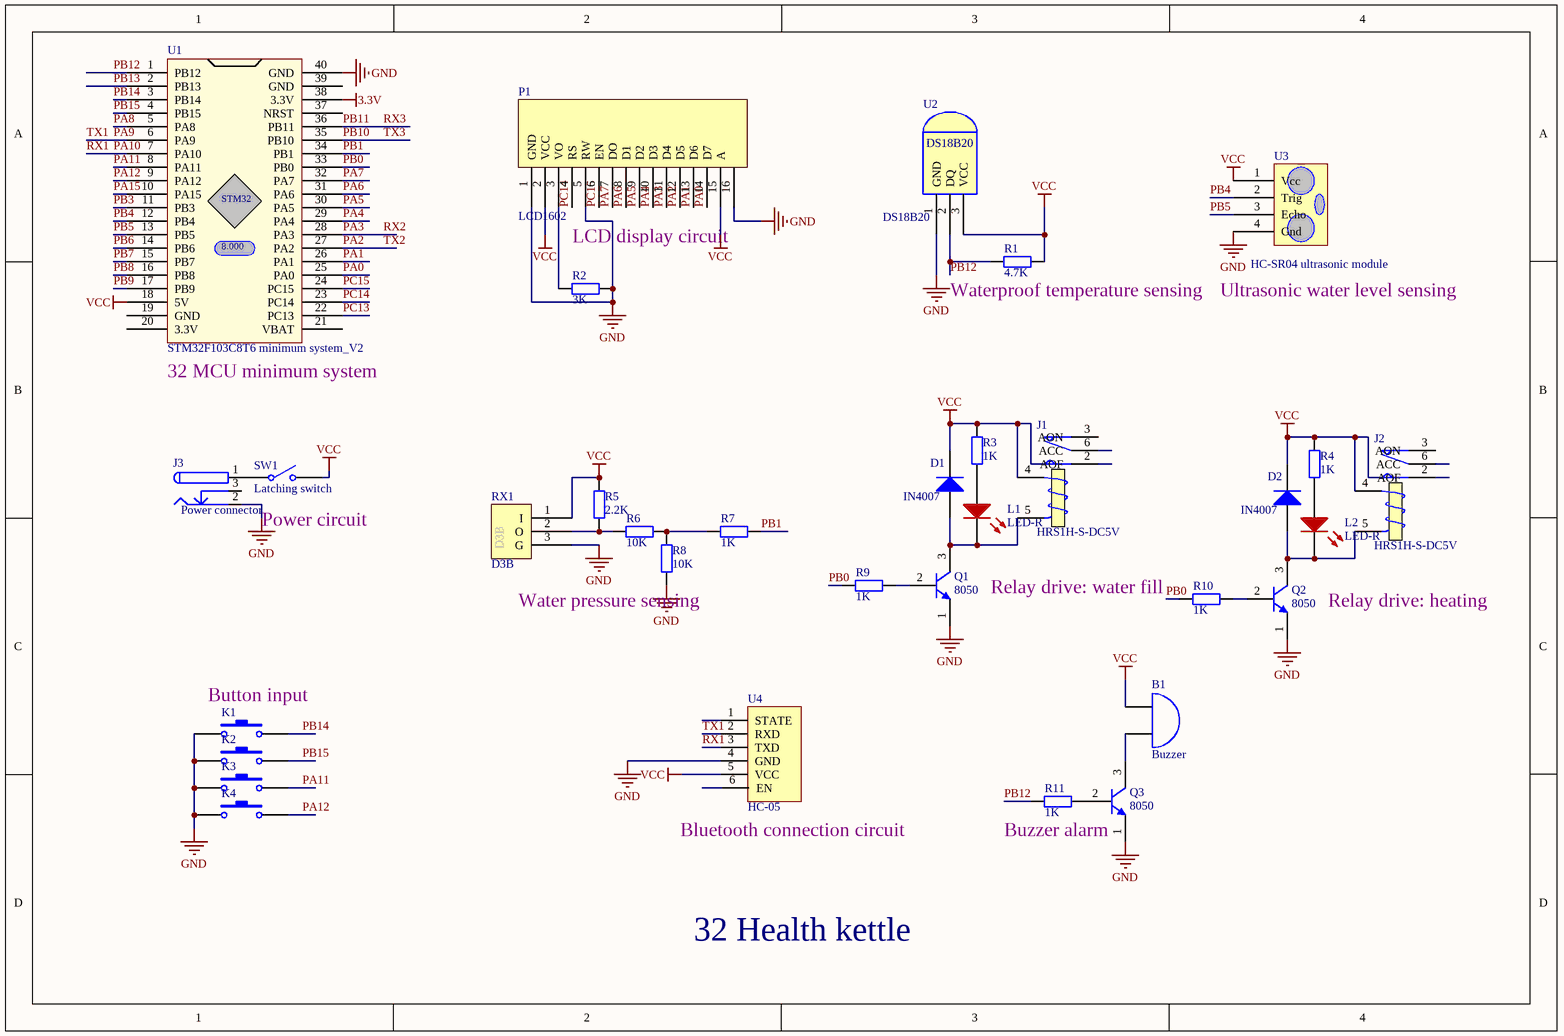
[diagram p0: MISC84237-2.SchDoc]
# Altium project MISC84237.PrjPcb
5 sheets, 81 parts. Net scope: global (net labels, ports and power ports of the same name join across sheets).
Board files: MISC84237-4.PcbDoc, MISC84237-7.PcbDoc, MISC84237.PcbDoc
Sheets:
  MISC84237-2.SchDoc
  MISC84237-3.SchDoc
  MISC84237-5.SchDoc
  MISC84237-6.SchDoc
  MISC84237-8.SchDoc

## Sheet MISC84237-2.SchDoc
size A4; PageSetup: Record=PageOptions|CenterHorizontal=True|CenterVertical=True|PrintScale=0.97|XCorrection=1.00|YCorrection=1.00|PrintKind=0|BorderSize=5000000|LeftOffset=0|BottomOffset=0|Orientation=2|PaperLength=1000|PaperWidth=1000|Scale=100|PaperSource=7|PrintQuality=-4|MediaType=1|DitherType=10|PaperKind=A4|PrintScaleMode=1

### Parts
(Parts that share a designator on the sheet are numbered #1, #2 ... from top to bottom, then left to right.)
B1  Buzzer  [Buzzy-Small]
D1#1  IN4007  [Diode-0.3]
D2#1  IN4007  [Diode-0.3]
J1#1  HRS1H-S-DC5V  [JDIANQI]
J2#1  HRS1H-S-DC5V  [JDIANQI]
J3#1  Power connector  [DC-JACK]
K1#1  Tactile button  [SW-6-6]  (value not drawn)
K2#1  Tactile button  [SW-6-6]  (value not drawn)
K3#1  Tactile button  [SW-6-6]  (value not drawn)
K4#1  Tactile button  [SW-6-6]  (value not drawn)
L1#1  LED-R  [LED-3]
L2#1  LED-R  [LED-3]
P1#1  LCD1602  [1602]
Q1#1  8050  [TO-92-2N3906]
Q2#1  8050  [TO-92-2N3906]
Q3#1  8050  [TO-92-2N3906]
R1#1  4.7K  [AXIAL-0.3]
R2#1  3K  [AXIAL-0.3]
R3#1  1K  [AXIAL-0.3]
R4#1  1K  [AXIAL-0.3]
R5#1  2.2K  [AXIAL-0.3]
R6#1  10K  [AXIAL-0.3]
R7#1  1K  [AXIAL-0.3]
R8#1  10K  [AXIAL-0.3]
R9#1  1K  [AXIAL-0.3]
R10#1  1K  [AXIAL-0.3]
R11#1  1K  [AXIAL-0.3]
RX1#1  D3B  [HDR1X3]
SW1#1  Latching switch  [SW1]
U1#1  STM32F103C8T6 minimum system_V2  [STM32F103C8T6_V2]
U2#1  DS18B20  [DS18b20]
U3#1  HC-SR04 ultrasonic module  [chaoshengbo-4]
U4#1  HC-05  [bluetooth]

### Nets
3.3V: U1#1.38(3.3V)
GND: J3#1.2 K1#1.1 K2#1.1 K3#1.1 K4#1.1 P1#1.1(GND) P1#1.5(RW) P1#1.16(K) Q1#1.1(E) Q2#1.1(E) Q3#1.1(E) R2#1.2 R8#1.1 RX1#1.3(G) U1#1.40(GND) U2#1.1(GND) U3#1.4(Gnd) U4#1.4(GND)
VCC: B1.1(A) D1#1.2(K) D2#1.2(K) J1#1.4(T1) J2#1.4(T1) P1#1.2(VCC) P1#1.15(A) R1#1.2 R3#1.2 R4#1.2 R5#1.2 RX1#1.1(I) SW1#1.2(NO) U1#1.18(5V) U2#1.3(VCC) U3#1.1(Vcc) U4#1.5(VCC)
PA0: P1#1.14(D7) U1#1.25(PA0)
PA1: P1#1.13(D6) U1#1.26(PA1)
PA2: P1#1.12(D5) U1#1.27(PA2)  [also labelled TX2]
PA3: P1#1.11(D4) U1#1.28(PA3)  [also labelled RX2]
PA4: P1#1.10(D3) U1#1.29(PA4)
PA5: P1#1.9(D2) U1#1.30(PA5)
PA6: P1#1.8(D1) U1#1.31(PA6)
PA7: P1#1.7(DO) U1#1.32(PA7)
PA8: U1#1.5(PA8)
PA9: U1#1.6(PA9) U4#1.2(RXD)  [also labelled TX1]
PA10: U1#1.7(PA10) U4#1.3(TXD)  [also labelled RX1]
PA11: K3#1.2 U1#1.8(PA11)
PA12: K4#1.2 U1#1.9(PA12)
PA15: U1#1.10(PA15)
PB0: R9#1.1 R10#1.1 U1#1.33(PB0)
PB1: R7#1.1 U1#1.34(PB1)
PB3: U1#1.11(PB3)
PB4: U1#1.12(PB4) U3#1.2(Trig)
PB5: U1#1.13(PB5) U3#1.3(Echo)
PB6: U1#1.14(PB6)
PB7: U1#1.15(PB7)
PB8: U1#1.16(PB8)
PB9: U1#1.17(PB9)
PB10: U1#1.35(PB10)  [also labelled TX3]
PB11: U1#1.36(PB11)  [also labelled RX3]
PB12: R1#1.1 R11#1.1 U1#1.1(PB12) U2#1.2(DQ)
PB13: U1#1.2(PB13)
PB14: K1#1.2 U1#1.3(PB14)
PB15: K2#1.2 U1#1.4(PB15)
PC13: U1#1.22(PC13)
PC14: P1#1.4(RS) U1#1.23(PC14)
PC15: P1#1.6(EN) U1#1.24(PC15)
NetB1_2: B1.2(B) Q3#1.3(C)
NetD1#1_1: D1#1.1(A) J1#1.5(T2) L1#1.2(K) Q1#1.3(C)
NetD2#1_1: D2#1.1(A) J2#1.5(T2) L2#1.2(K) Q2#1.3(C)
NetJ3#1_1: J3#1.1 SW1#1.1(COMMON)
NetL1#1_1: L1#1.1(A) R3#1.1
NetL2#1_1: L2#1.1(A) R4#1.1
NetP1#1_3: P1#1.3(VO) R2#1.1
NetQ1#1_2: Q1#1.2(B) R9#1.2
NetQ2#1_2: Q2#1.2(B) R10#1.2
NetQ3#1_2: Q3#1.2(B) R11#1.2
NetR5#1_1: R5#1.1 R6#1.1 RX1#1.2(O)
NetR6#1_2: R6#1.2 R7#1.2 R8#1.2

Not connected (* = marked no-connect by the designer): J1#1 2(AOF) 3(AON) 6(ACC); J2#1 2(AOF) 3(AON) 6(ACC); J3#1 3; U1#1 19(GND) 20(3.3V) 21(VBAT) 37(NRST) 39(GND); U4#1 1(STATE) 6(EN)

### Notes on the sheet
- LCD display circuit
- (near R1#1) Waterproof temperature sensing
- (near U3#1) Ultrasonic water level sensing
- (near U1#1) 32 MCU minimum system
- Power circuit
- (near R8#1) Water pressure sensing
- (near R10#1) Relay drive: water fill
- Relay drive: heating
- (near K1#1) Button input
- (near U4#1) Bluetooth connection circuit
- (near Q3#1) Buzzer alarm
- 32 Health kettle

### Library data of the parts
B1 = Bell: Electrical Bell; Value: 5V  有源蜂鸣器; Published: 24-Mar-1999; LatestRevisionDate: 17-Jul-2002; LatestRevisionNote: Re-released for DXP Platform.; PackageReference: PIN2; Publisher: Altium Limited
D1#1 D2#1 = DIODE: Value: IN4007二极管
J1#1 J2#1 = jidianqi: Value: HK4100F-DC5V-SHG 继电器（5V黄色6腿继电器）
J3#1 = DC002: Low Voltage Power Supply Connector; Value: DC-002电源插座 3.5-1.1MM DC电源座; Published: 17-Dec-2003; DatasheetDocument: 09-May-2002; ComponentLink1Description: Manufacturer Link; ComponentLink1URL: http://domino.kycon.com/internet/Products.html; Publisher: Altium Limited
K1#1 K2#1 K3#1 K4#1 = SW-AJ: Value: 轻触按键
L1#1 L2#1 = LED-R: Value: 3mm红色LED灯
P1#1 = LCD1602: Value: LCD1602液晶显示+16P排座
Q1#1 Q2#1 Q3#1 = 8050: Value: 8050三极管
R1#1 = RES2: Resistor; Value: 4.7K电阻
R2#1 = Res2: Resistor; Value: 3K电阻
R3#1 R4#1 = Res2: Resistor; Value: 1K电阻
R5#1 = RES2: Resistor; Value: 2.2K电阻
R6#1 R8#1 = RES2: Resistor; Value: 10K电阻
R7#1 = RES0.4: Value: 1K电阻
R9#1 R10#1 R11#1 = RES2: Resistor; Value: 1K电阻
RX1#1 = D3B: Value: D3B压力传感器+瓶盖
SW1#1 = SW-SPST: Value: 自锁开关
U1#1 = STM32F103C8T6最小系统_V2
U2#1 = DS18B20: Value: 防水DS18B20温度传感器
U3#1 = HC-SR04: Value: HC-SR04  超声波模块
U4#1 = Bluetooth: Value: 蓝牙 HC-05模块+6P排座

## Sheet MISC84237-3.SchDoc
size A3; PageSetup: Record=PageOptions¦CenterHorizontal=True¦CenterVertical=True¦PrintScale=0.97¦XCorrection=1.00¦YCorrection=1.00¦PrintKind=0¦BorderSize=5000000¦LeftOffset=0¦BottomOffset=0¦Orientation=2¦PaperLength=1000¦PaperWidth=1000¦Scale=100¦PaperSource=7¦PrintQuality=-4¦MediaType=1¦DitherType=10¦PaperKind=A4¦PrintScaleMode=1
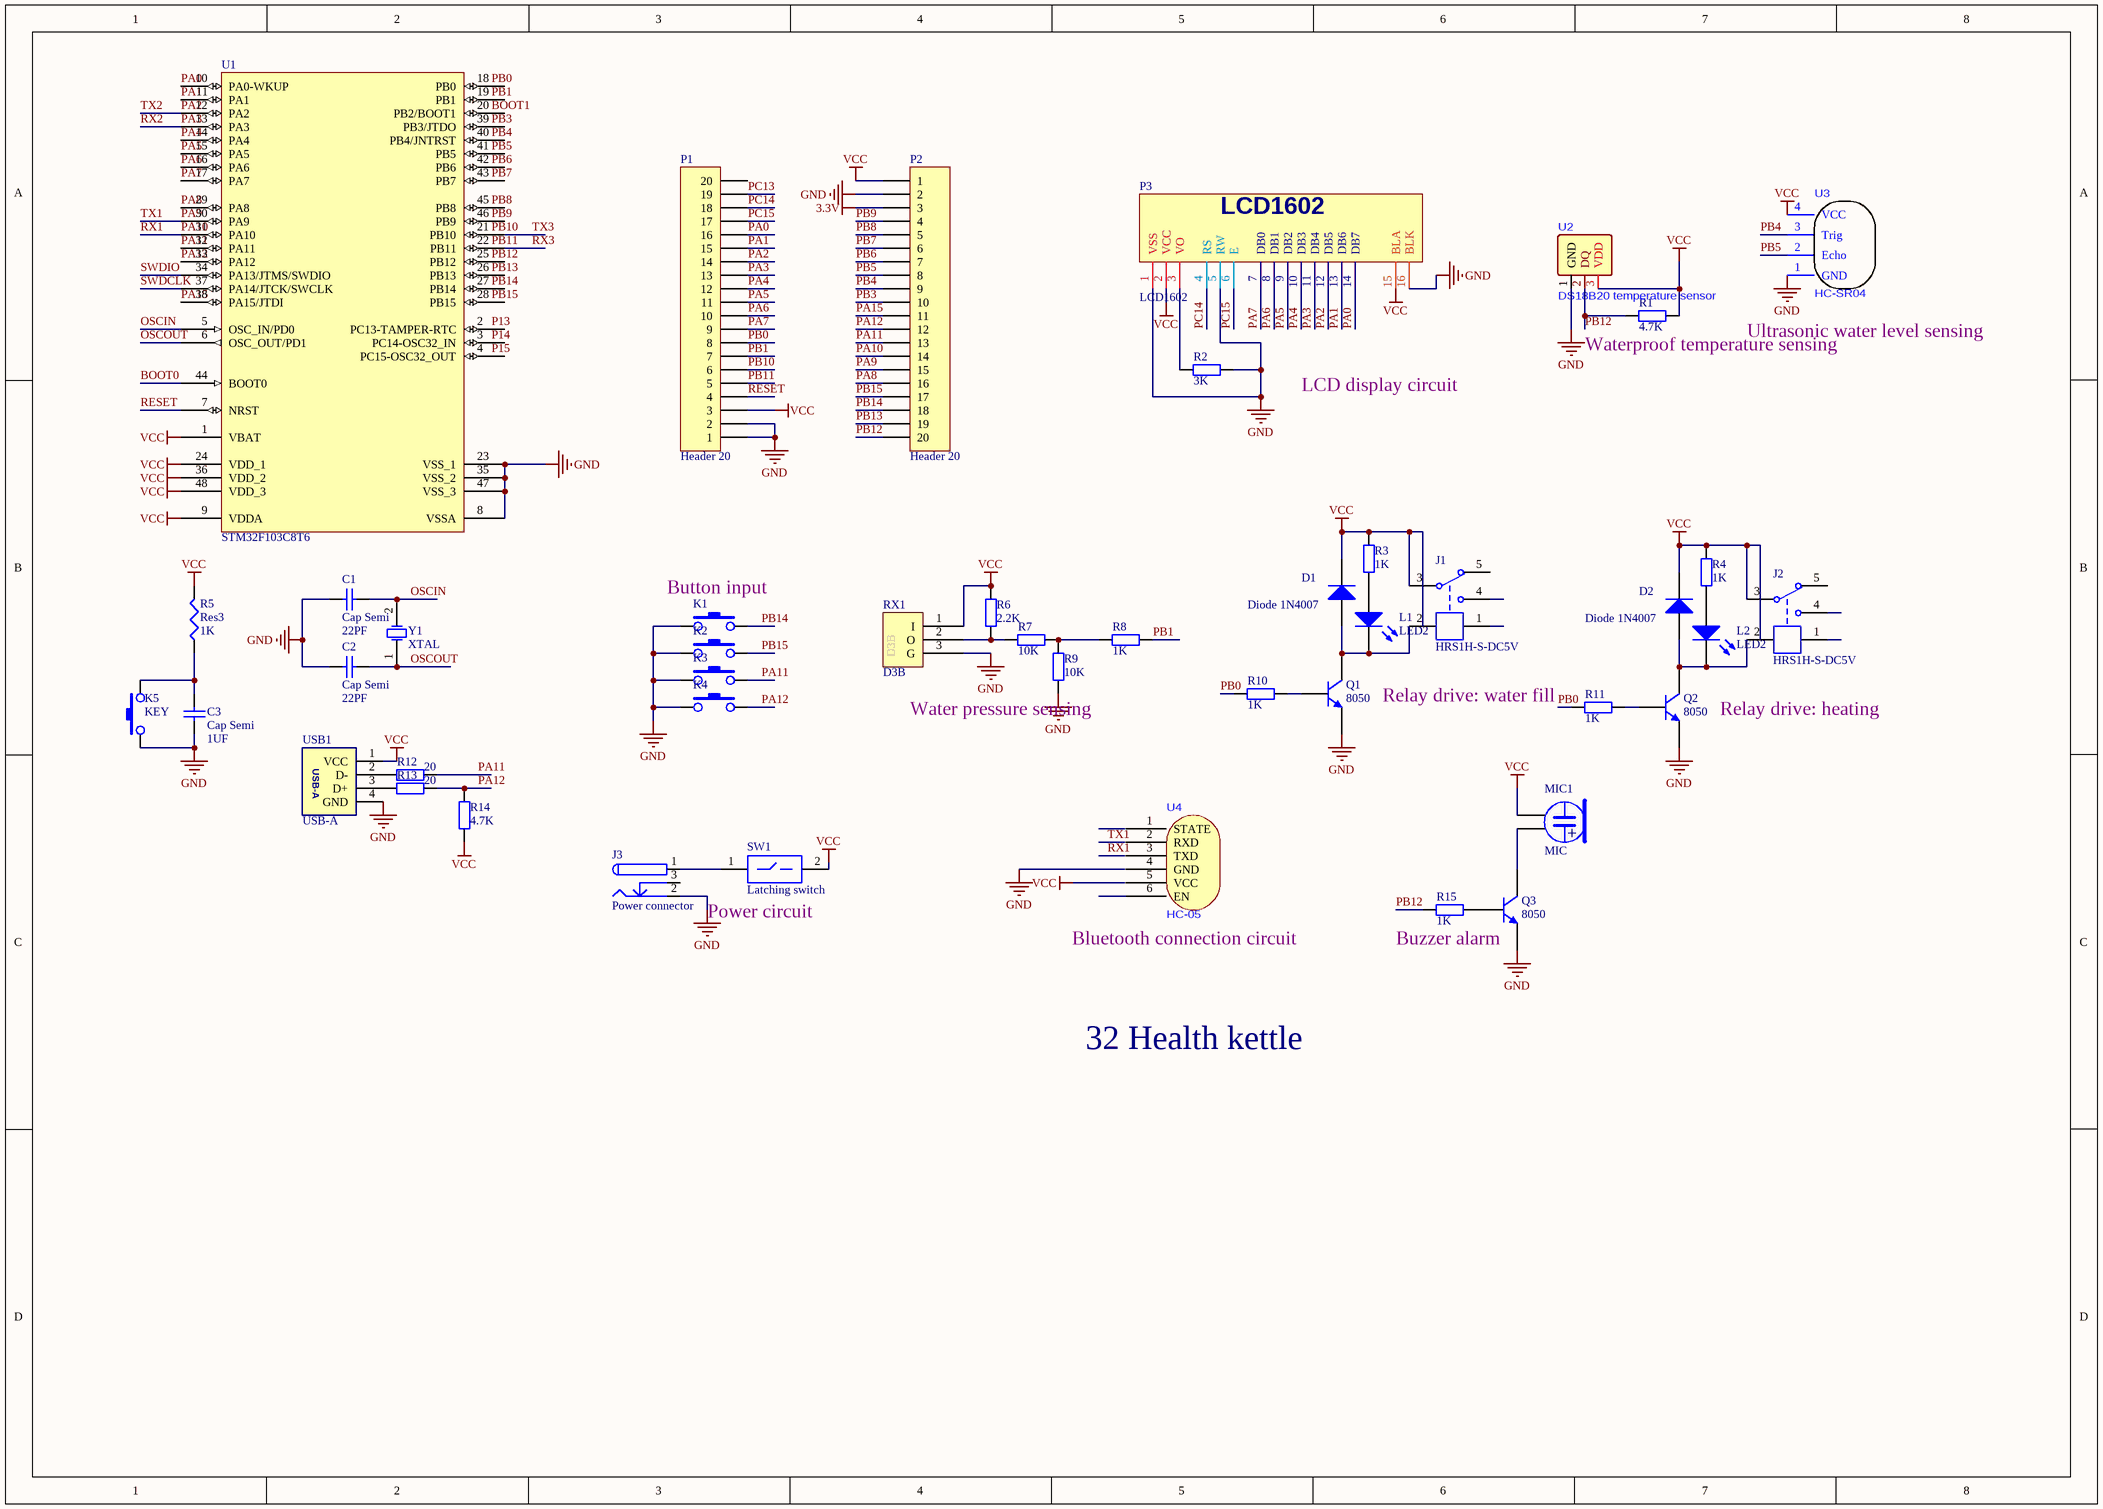
[diagram p1: MISC84237-3.SchDoc]

### Parts
(Parts that share a designator on the sheet are numbered #1, #2 ... from top to bottom, then left to right.)
C1  Cap Semi  value 22PF  [C1206]
C2  Cap Semi  value 22PF  [C1206]
C3  Cap Semi  value 1UF  [C1206]
D1#2  Diode 1N4007  [DO-41]
D2#2  Diode 1N4007  [DO-41]
J1#2  HRS1H-S-DC5V  [HRS1H]
J2#2  HRS1H-S-DC5V  [HRS1H]
J3#2  Power connector  [DC-002]
K1#2  KEY  [DIP-3X6X4.3]  (value not drawn)
K2#2  KEY  [DIP-3X6X4.3]  (value not drawn)
K3#2  KEY  [DIP-3X6X4.3]  (value not drawn)
K4#2  KEY  [DIP-3X6X4.3]  (value not drawn)
K5  KEY  [DIP-3X6X4.3]
L1#2  LED2  [3.2X1.6X1.1]
L2#2  LED2  [3.2X1.6X1.1]
MIC1  MIC  [MIC-4.5X1.9]
P1#2  Header 20  [HDR1X20]
P2  Header 20  [HDR1X20]
P3  LCD1602  [LCD1602]
Q1#2  8050  [TO-226-AA]
Q2#2  8050  [TO-226-AA]
Q3#2  8050  [TO-226-AA]
R1#2  4.7K  [AXIAL-0.3]
R2#2  3K  [AXIAL-0.3]
R3#2  1K  [AXIAL-0.3]
R4#2  1K  [AXIAL-0.3]
R5#2  Res3  value 1K  [J1-0603]
R6#2  2.2K  [AXIAL-0.3]
R7#2  10K  [AXIAL-0.3]
R8#2  1K  [AXIAL-0.3]
R9#2  10K  [AXIAL-0.3]
R10#2  1K  [AXIAL-0.3]
R11#2  1K  [AXIAL-0.3]
R12  20  [AXIAL-0.3]
R13  20  [AXIAL-0.3]
R14  4.7K  [AXIAL-0.3]
R15  1K  [AXIAL-0.3]
RX1#2  D3B  [HDR1X3]
SW1#2  Latching switch  [DIP-1P]
U1#2  STM32F103C8T6  [LQFP48_N]
U2#2  DS18B20 temperature sensor  [DS18B20温度传感器]
U3#2  HC-SR04  [HC-SR04]
U4#2  HC-05  [HC-05]
USB1  USB-A  [USB-A/S_A]
Y1  XTAL  [R38]

### Nets
3.3V: P2.3
GND: C1.2 C2.2 C3.1 J3#2.2 K1#2.1 K2#2.1 K3#2.1 K4#2.1 K5.1 P1#2.1 P1#2.2 P2.2 P3.1(VSS) P3.5(RW) P3.16(BLK) Q1#2.3(E) Q2#2.3(E) Q3#2.3(E) R2#2.2 R9#2.1 RX1#2.3(G) U1#2.8(VSSA) U1#2.23(VSS_1) U1#2.35(VSS_2) U1#2.47(VSS_3) U2#2.1(GND) U3#2.1(GND) USB1.4(GND)
VCC: D1#2.2(K) D2#2.2(K) J1#2.3 J2#2.3 MIC1.2 P1#2.3 P2.1 P3.2(VCC) P3.15(BLA) R1#2.2 R3#2.2 R4#2.2 R5#2.2 R6#2.2 R14.2 RX1#2.1(I) SW1#2.2 U1#2.1(VBAT) U1#2.9(VDDA) U1#2.24(VDD_1) U1#2.36(VDD_2) U1#2.48(VDD_3) U2#2.3(VDD) U3#2.4(VCC) USB1.1(VCC)
BOOT0: U1#2.44(BOOT0)
OSCIN: C1.1 U1#2.5(OSC_IN/PD0) Y1.2(OSC2)
OSCOUT: C2.1 U1#2.6(OSC_OUT/PD1) Y1.1(OSC1)
PA0: P1#2.16 P3.14(DB7) U1#2.10(PA0-WKUP)
PA1: P1#2.15 P3.13(DB6) U1#2.11(PA1)
PA2: P1#2.14 P3.12(DB5) U1#2.12(PA2)  [also labelled TX2]
PA3: P1#2.13 P3.11(DB4) U1#2.13(PA3)  [also labelled RX2]
PA4: P1#2.12 P3.10(DB3) U1#2.14(PA4)
PA5: P1#2.11 P3.9(DB2) U1#2.15(PA5)
PA6: P1#2.10 P3.8(DB1) U1#2.16(PA6)
PA7: P1#2.9 P3.7(DB0) U1#2.17(PA7)
PA8: P2.16 U1#2.29(PA8)
PA9: P2.15 U1#2.30(PA9)  [also labelled TX1]
PA10: P2.14 U1#2.31(PA10)  [also labelled RX1]
PA11: K3#2.3 P2.13 R12.1 U1#2.32(PA11)
PA12: K4#2.3 P2.12 R13.1 R14.1 U1#2.33(PA12)
PA15: P2.11 U1#2.38(PA15/JTDI)
PB0: P1#2.8 R10#2.1 R11#2.1
PB1: P1#2.7 R8#2.1
PB3: P2.10
PB4: P2.9 U3#2.3(Trig)
PB5: P2.8 U3#2.2(Echo)
PB6: P2.7
PB7: P2.6
PB8: P2.5
PB9: P2.4
PB10: P1#2.6 U1#2.21(PB10)  [also labelled TX3]
PB11: P1#2.5 U1#2.22(PB11)  [also labelled RX3]
PB12: P2.20 R1#2.1 R15.1 U2#2.2(DQ)
PB13: P2.19
PB14: K1#2.3 P2.18
PB15: K2#2.3 P2.17
PC13: P1#2.19
PC14: P1#2.18 P3.4(RS)
PC15: P1#2.17 P3.6(E)
RESET: P1#2.4 U1#2.7(NRST)
SWDCLK: U1#2.37(PA14/JTCK/SWCLK)
SWDIO: U1#2.34(PA13/JTMS/SWDIO)
NetC3_2: C3.2 K5.3 R5#2.1
NetD1#2_1: D1#2.1(A) J1#2.2 L1#2.2(K) Q1#2.1(C)
NetD2#2_1: D2#2.1(A) J2#2.2 L2#2.2(K) Q2#2.1(C)
NetJ3#2_1: J3#2.1 SW1#2.1(A1)
NetL1#2_1: L1#2.1(A) R3#2.1
NetL2#2_1: L2#2.1(A) R4#2.1
NetMIC1_1: MIC1.1 Q3#2.1(C)
NetP3_3: P3.3(VO) R2#2.1
NetQ1#2_2: Q1#2.2(B) R10#2.2
NetQ2#2_2: Q2#2.2(B) R11#2.2
NetQ3#2_2: Q3#2.2(B) R15.2
NetR6#2_1: R6#2.1 R7#2.1 RX1#2.2(O)
NetR7#2_2: R7#2.2 R8#2.2 R9#2.2
NetR12_2: R12.2 USB1.2(D-)
NetR13_2: R13.2 USB1.3(D+)

Not connected (* = marked no-connect by the designer): J1#2 1 4 5; J2#2 1 4 5; J3#2 3; P1#2 20; U1#2 2(PC13-TAMPER-RTC) 3(PC14-OSC32_IN) 4(PC15-OSC32_OUT) 18(PB0) 19(PB1) 20(PB2/BOOT1) 25(PB12) 26(PB13) 27(PB14) 28(PB15) 39(PB3/JTDO) 40(PB4/JNTRST) 41(PB5) 42(PB6) 43(PB7) 45(PB8) 46(PB9); U4#2 1(STATE) 2(RXD) 3(TXD) 4(GND) 5(VCC) 6(EN)

### Notes on the sheet
- (near R1#2) Waterproof temperature sensing
- (near U3#2) Ultrasonic water level sensing
- LCD display circuit
- (near K1#2) Button input
- (near R9#2) Water pressure sensing
- (near R11#2) Relay drive: water fill
- Relay drive: heating
- Power circuit
- (near U4#2) Bluetooth connection circuit
- (near Q3#2) Buzzer alarm
- 32 Health kettle
- Labels drawn without touching a wire or pin: BOOT1, P13, P14, P15, PB0, PB1, PB3, PB4, PB5, PB6, PB7, PB8, PB9, PB10, PB11, PB12, PB13, PB14, PB15

### Library data of the parts
C1-C3 = Cap Semi: Capacitor (Semiconductor SIM Model); Published: 8-Jun-2000; LatestRevisionDate: 29-May-2009; LatestRevisionNote: IPC-7351 Footprint Added.; PackageReference: C1206; PackageDescription: Chip Capacitor; Publisher: Altium Limited
D1#2 D2#2 = Diode 1N4007: 1 Amp General Purpose Rectifier; Published: 8-Jun-2000; LatestRevisionDate: 17-Jul-2002; LatestRevisionNote: Re-released for DXP Platform.; DatasheetVersion: 1998; PackageVersion: Aug-1999; PackageReference: DO-41; PackageDescription: Diode, Axial; Body 5.2 x 2.7 mm (LxDia. max), Lead Dia. 0.86 mm (max); Code_JEDEC: DO-204-AL; ComponentLink1Description: Manufacturer Link; ComponentLink1URL: http://www.fairchildsemi.com/; ComponentLink2Description: Datasheet; ComponentLink2URL: http://www.fairchildsemi.com/ds/1N%2F1N4001.pdf; Publisher: Altium Limited
J1#2 J2#2 = HRS1H-S-DC5V: 5V SPDT changeover
J3#2 = DC_Socket
L1#2 L2#2 = LED2: Typical RED, GREEN, YELLOW, AMBER GaAs LED; Published: 8-Jun-2000; LatestRevisionDate: 17-Jul-2002; LatestRevisionNote: Re-released for DXP Platform.; PackageVersion: Feb-2002; PackageReference: 3.2X1.6X1.1; PackageDescription: SM LED; 2 Flat Leads; Publisher: Altium Limited
MIC1 = MIC: Condenser microphone
P1#2 P2 = Header 20: Header, 20-Pin; LatestRevisionDate: 17-Jul-2002; LatestRevisionNote: Re-released for DXP Platform.; Publisher: Altium Limited
Q1#2 Q2#2 Q3#2 = NPN: NPN Bipolar Transistor; Published: 8-Jun-2000; LatestRevisionDate: 17-Jul-2002; LatestRevisionNote: Re-released for DXP Platform.; PackageReference: TO-226-AA; PackageDescription: TO, Flat Index; 3 In-Line, Axial Leads; Body Dia. 4.8mm; Leads 0.55 x 0.51 mm (max); Code_JEDEC: TO-226-AA; Publisher: Altium Limited
R1#2 = RES2: Resistor; Value: 4.7K电阻
R2#2 = Res2: Resistor; Value: 3K电阻
R3#2 R4#2 = Res2: Resistor; Value: 1K电阻
R5#2 = Res3: Resistor; Published: 8-Jun-2000; LatestRevisionDate: 29-May-2009; LatestRevisionNote: IPC-7351 Footprint Added.; PackageReference: J1-0603; PackageDescription: Chip Resistor; Publisher: Altium Limited
R6#2 R12-R14 = RES2: Resistor; Value: 2.2K电阻
R7#2 R9#2 = RES2: Resistor; Value: 10K电阻
R8#2 = RES0.4: Value: 1K电阻
R10#2 R11#2 R15 = RES2: Resistor; Value: 1K电阻
RX1#2 = D3B: Value: D3B压力传感器+瓶盖
SW1#2 = SW1-DIP2
U1#2 = STM32F103C8T6: STM32 ARM-based 32-bit MCU with 64 Kbytes Flash, 48-pin LQFP, Industrial Temperature; Published: 30-May-2008; DatasheetVersion: rev6, Mar-2008; PackageVersion: Mar-2008; PackageReference: LQFP48; PackageDescription: 48-Pin Low-Profile Quad Flat Pack, 7 x 7 mm Body, 0.5 mm Pitch (LQFP48); ComponentLink1Description: Manufacturer Link; ComponentLink1URL: www.st.com/stm32; ComponentLink2Description: Datasheet; ComponentLink2URL: http://www.st.com/stonline/products/literature/ds/13587.pdf; Publisher: Altium Limited
U2#2 = DS18B20温度传感器
U3#2 = HC
Y1 = XTAL: Crystal Oscillator; Published: 8-Jun-2000; LatestRevisionDate: 17-Jul-2002; LatestRevisionNote: Re-released for DXP Platform.; PackageReference: R38; PackageDescription: Crystal, Thru-Hole; 2 Leads; Body 3.1 x 8.2 mm (Dia.xH); Publisher: Altium Limited

## Sheet MISC84237-5.SchDoc
size 41 x 32 mm
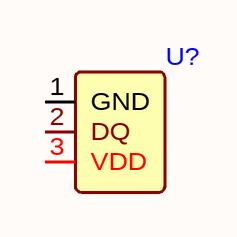
[diagram p2: MISC84237-5.SchDoc]

### Parts
(Parts that share a designator on the sheet are numbered #1, #2 ... from top to bottom, then left to right.)
U?#1  (no value)  [DS18B20温度传感器]

### Nets

Not connected (* = marked no-connect by the designer): U?#1 1(GND) 2(DQ) 3(VDD)

### Library data of the parts
U?#1 = DS18B20温度传感器

## Sheet MISC84237-6.SchDoc
size 49 x 40 mm
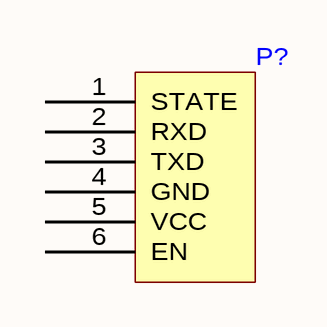
[diagram p3: MISC84237-6.SchDoc]

### Parts
P?  (no value)  [HC-05]

### Nets

Not connected (* = marked no-connect by the designer): P? 1(STATE) 2(RXD) 3(TXD) 4(GND) 5(VCC) 6(EN)

### Library data of the parts
P? = HC-05

## Sheet MISC84237-8.SchDoc
size 48 x 39 mm
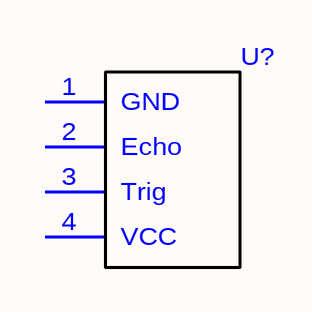
[diagram p4: MISC84237-8.SchDoc]

### Parts
(Parts that share a designator on the sheet are numbered #1, #2 ... from top to bottom, then left to right.)
U?#2  (no value)  [HC-SR04]

### Nets

Not connected (* = marked no-connect by the designer): U?#2 1(GND) 2(Echo) 3(Trig) 4(VCC)

### Library data of the parts
U?#2 = HC-SR04

## Nets that join several sheets
3.3V: MISC84237-2 (U1#1.38), MISC84237-3 (P2.3)
GND: MISC84237-2 (18 pins), MISC84237-3 (28 pins)
VCC: MISC84237-2 (17 pins), MISC84237-3 (25 pins)
PA0: MISC84237-2 (P1#1.14 U1#1.25), MISC84237-3 (P1#2.16 P3.14 U1#2.10)
PA1: MISC84237-2 (P1#1.13 U1#1.26), MISC84237-3 (P1#2.15 P3.13 U1#2.11)
PA2: MISC84237-2 (P1#1.12 U1#1.27), MISC84237-3 (P1#2.14 P3.12 U1#2.12)
PA3: MISC84237-2 (P1#1.11 U1#1.28), MISC84237-3 (P1#2.13 P3.11 U1#2.13)
PA4: MISC84237-2 (P1#1.10 U1#1.29), MISC84237-3 (P1#2.12 P3.10 U1#2.14)
PA5: MISC84237-2 (P1#1.9 U1#1.30), MISC84237-3 (P1#2.11 P3.9 U1#2.15)
PA6: MISC84237-2 (P1#1.8 U1#1.31), MISC84237-3 (P1#2.10 P3.8 U1#2.16)
PA7: MISC84237-2 (P1#1.7 U1#1.32), MISC84237-3 (P1#2.9 P3.7 U1#2.17)
PA8: MISC84237-2 (U1#1.5), MISC84237-3 (P2.16 U1#2.29)
PA9: MISC84237-2 (U1#1.6 U4#1.2), MISC84237-3 (P2.15 U1#2.30)
PA10: MISC84237-2 (U1#1.7 U4#1.3), MISC84237-3 (P2.14 U1#2.31)
PA11: MISC84237-2 (K3#1.2 U1#1.8), MISC84237-3 (K3#2.3 P2.13 R12.1 U1#2.32)
PA12: MISC84237-2 (K4#1.2 U1#1.9), MISC84237-3 (5 pins)
PA15: MISC84237-2 (U1#1.10), MISC84237-3 (P2.11 U1#2.38)
PB0: MISC84237-2 (R9#1.1 R10#1.1 U1#1.33), MISC84237-3 (P1#2.8 R10#2.1 R11#2.1)
PB1: MISC84237-2 (R7#1.1 U1#1.34), MISC84237-3 (P1#2.7 R8#2.1)
PB3: MISC84237-2 (U1#1.11), MISC84237-3 (P2.10)
PB4: MISC84237-2 (U1#1.12 U3#1.2), MISC84237-3 (P2.9 U3#2.3)
PB5: MISC84237-2 (U1#1.13 U3#1.3), MISC84237-3 (P2.8 U3#2.2)
PB6: MISC84237-2 (U1#1.14), MISC84237-3 (P2.7)
PB7: MISC84237-2 (U1#1.15), MISC84237-3 (P2.6)
PB8: MISC84237-2 (U1#1.16), MISC84237-3 (P2.5)
PB9: MISC84237-2 (U1#1.17), MISC84237-3 (P2.4)
PB10: MISC84237-2 (U1#1.35), MISC84237-3 (P1#2.6 U1#2.21)
PB11: MISC84237-2 (U1#1.36), MISC84237-3 (P1#2.5 U1#2.22)
PB12: MISC84237-2 (R1#1.1 R11#1.1 U1#1.1 U2#1.2), MISC84237-3 (P2.20 R1#2.1 R15.1 U2#2.2)
PB13: MISC84237-2 (U1#1.2), MISC84237-3 (P2.19)
PB14: MISC84237-2 (K1#1.2 U1#1.3), MISC84237-3 (K1#2.3 P2.18)
PB15: MISC84237-2 (K2#1.2 U1#1.4), MISC84237-3 (K2#2.3 P2.17)
PC13: MISC84237-2 (U1#1.22), MISC84237-3 (P1#2.19)
PC14: MISC84237-2 (P1#1.4 U1#1.23), MISC84237-3 (P1#2.18 P3.4)
PC15: MISC84237-2 (P1#1.6 U1#1.24), MISC84237-3 (P1#2.17 P3.6)